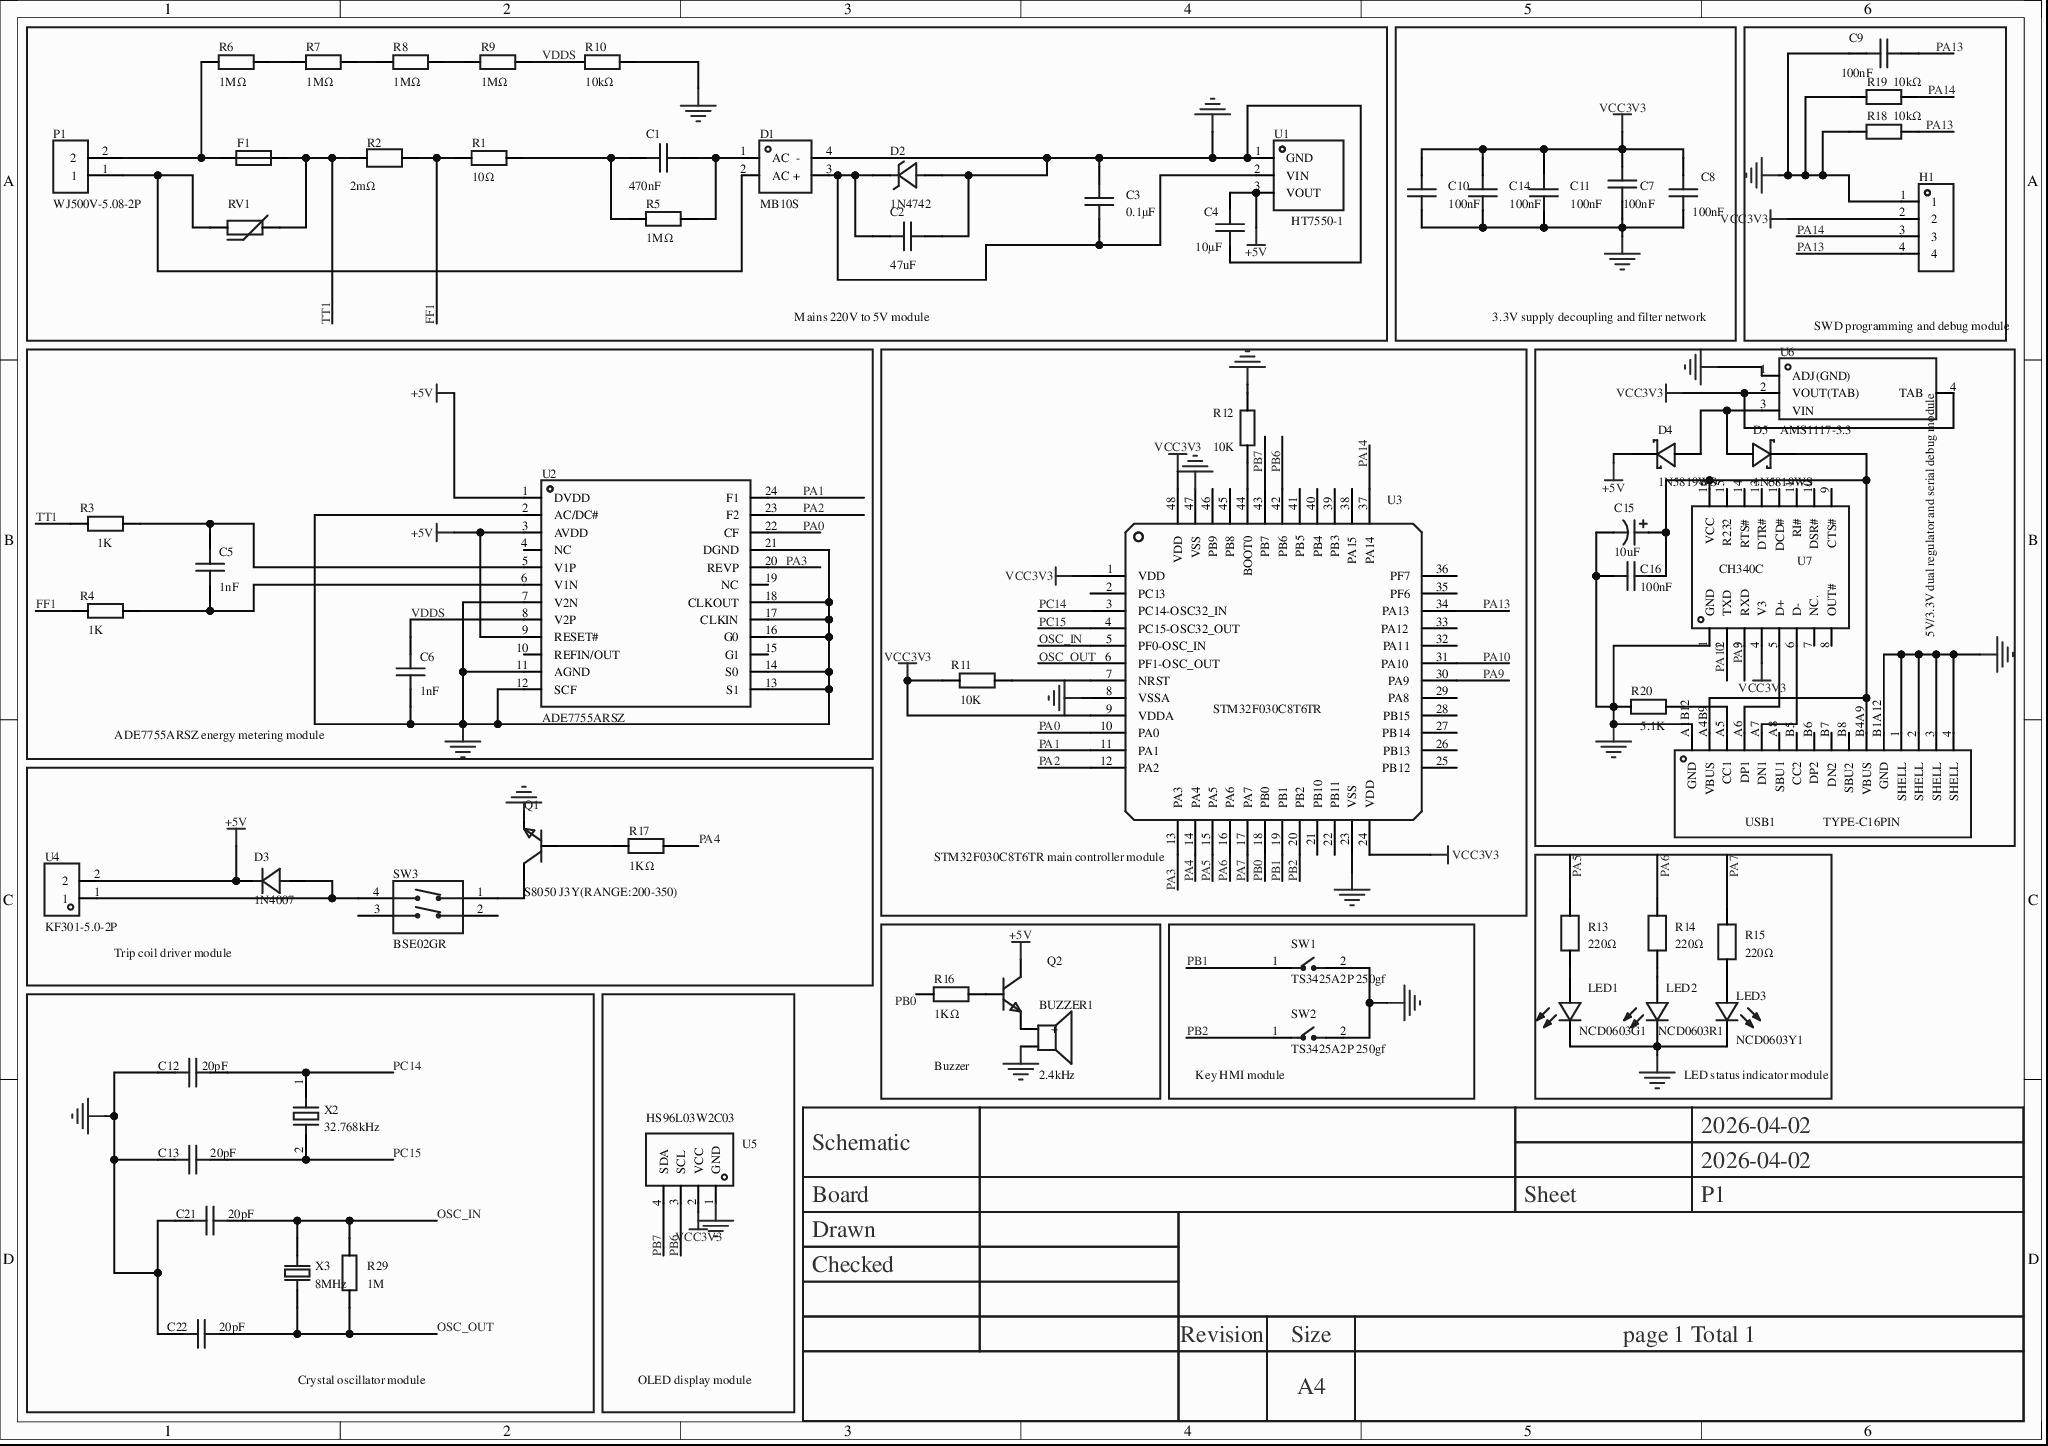
[diagram p0: MISC61242-3.schdoc]
# Altium project MISC61242-2.PrjPcb
1 sheet, 67 parts. Net scope: global (net labels, ports and power ports of the same name join across sheets).
Board file: MISC61242.pcbdoc

## Sheet MISC61242-3.schdoc
size 297 x 209 mm; Version: V1.0; @Project Name: MISC61242; @Update Date: 2026-04-13; @Create Date: 2026-04-13; @Board Name: MISC61242; @Create Time: 14:55:17; @Page Count: 1; @Page No: 1; @Schematic Name: MISC61242; @Update Time: 14:55:17; Size: A4

### Parts
BUZZER1  2.4kHz  [BUZ-TH_BD12.0-P7.60-D0.6-FD]
C1  470nF  [CAP-TH_L17.0-W5.5-P15.00-D1.2]
C2  47uF  [C0603]
C3  0.1μF  [C0603]
C4  10μF  [C0603]
C5  1nF  [C0603]
C6  1nF  [C0603]
C7  100nF  [C0805]
C8  100nF  [C0805]
C9  100nF  [C0603]
C10  100nF  [C0805]
C11  100nF  [C0603]
C12  20pF  [C0805]
C13  20pF  [C0805]
C14  100nF  [C0805]
C15  10uF  [CAP-SMD_BD5.0-L5.3-W5.3-FD]
C16  100nF  [C0603]
C21  20pF  [C0805]
C22  20pF  [C0805]
D1  MB10S  [MBS_L4.7-W4.0-P2.50-LS7.0-TL]
D2  1N4742  [DO-41_BD2.4-L4.7-P8.70-D0.8-FD]
D3  1N4007  [SMA_L4.3-W2.5-LS5.0-RD]
D4  1N5819WS  [SOD-323_L1.8-W1.3-LS2.5-RD]
D5  1N5819WS  [SOD-323_L1.8-W1.3-LS2.5-RD]
F1  2F.0500212000S1B02  [FUSE-TH_BD3.0-L7.2-P11.20-D0.6]  (value not drawn)
H1  (no value)  [HDR-TH_4P-P2.54-V-F]
LED1  NCD0603G1  [LED0603-RD_1]
LED2  NCD0603R1  [LED0603-RD_RED]
LED3  NCD0603Y1  [LED0603-RD]
P1  WJ500V-5.08-2P  [CONN-TH_2P-P5.00_WJ500V-5.08-2P]
Q1  S8050 J3Y(RANGE:200-350)  [SOT-23-3_L3.0-W1.7-P0.95-LS2.9-BR]
Q2  (no value)  [S8050_SOT-23]
R1  10Ω  [R0603]
R2  2mΩ  [RES-SMD_L6.4-W3.2-1]
R3  1K  [R0603]
R4  1K  [R0603]
R5  1MΩ  [R0603]
R6  1MΩ  [R1206]
R7  1MΩ  [R1206]
R8  1MΩ  [R1206]
R9  1MΩ  [R1206]
R10  10kΩ  [R0805]
R11  10K  [R0603]
R12  10K  [R0603]
R13  220Ω  [R0402]
R14  220Ω  [R0402]
R15  220Ω  [R0402]
R16  1KΩ  [R0603]
R17  1KΩ  [R0603]
R18  10kΩ  [R0805]
R19  10kΩ  [R0805]
R20  5.1K  [R0603]
R29  1M  [R0805]
RV1  190pF@1kHz  [RES-TH_L12.5-W6.7-P7.50-D1.2]  (value not drawn)
SW1  TS3425A2P 250gf  [SW-SMD_L3.9-W2.9-LS5.0]
SW2  TS3425A2P 250gf  [SW-SMD_L3.9-W2.9-LS5.0]
SW3  BSE02GR  [SW-TH_4P-L9.9-W6.8-P7.62-BL]
U1  HT7550-1  [SOT-89_L4.5-W2.5-P1.50-LS4.2-BR]
U2  ADE7755ARSZ  [SSOP-24_L8.1-W5.3-P0.65-LS7.8-BL]
U3  STM32F030C8T6TR  [LQFP-48_L7.0-W7.0-P0.50-LS9.0-BL]
U4  KF301-5.0-2P  [HDR-M-2.54_1X2]
U5  HS96L03W2C03  [OLED-TH_L27.8-W27.2-P2.54_C9900033791]
U6  AMS1117-3.3  [SOT-223-4_L6.5-W3.5-P2.30-LS7.0-BR]
U7  CH340C  [SOP-16_L10.0-W3.9-P1.27-LS6.0-BL]
USB1  TYPE-C16PIN  [USB-C-SMD_TYPE-C16PIN]
X2  32.768kHz  [CRYSTAL-SMD_L3.2-W1.5-FC-135R32.7680KF-A3]
X3  8MHz  [CRYSTAL-SMD_L3.2-W2.5_3225-8MHZ]

### Blocks framed on the sheet
Mains 220V to 5V module: C1-C4 D1 D2 F1 P1 R1 R2 R5-R10 RV1 U1
3.3V supply decoupling and filter network: C7 C8 C10 C11 C14
SWD programming and debug module: C9 H1 R18 R19
ADE7755ARSZ energy metering module: C5 C6 R3 R4 U2
STM32F030C8T6TR main controller module: R11 R12 U3
5V/3.3V dual regulator and serial debug module: C15 C16 D4 D5 R20 U6 U7 USB1
Trip coil driver module: D3 Q1 R17 SW3 U4
LED status indicator module: LED1-LED3 R13-R15
Buzzer: BUZZER1 Q2 R16
Key HMI module: SW1 SW2
Crystal oscillator module: C12 C13 C21 C22 R29 X2 X3
OLED display module: U5

### Nets
+5V: C4.2 D3.1(K) D4.1(K) Q2.3 U1.3(VOUT) U2.1(DVDD) U2.3(AVDD) U2.9(RESET#) U4.2
GND: BUZZER1.2 C2.2 C3.2 C4.1 C6.1 C7.2 C8.1 C9.1 C10.2 C11.1 C12.2 C13.1 C14.1 C15.2 C16.1 C21.1 C22.1 D1.4(-) D2.1(A) H1.1 LED1.1(K) LED2.1(K) LED3.1(K) Q1.2(E) R10.2 R12.2 R18.2 R19.2 R20.2 SW1.2 SW2.2 U1.1(GND) U2.2(AC/DC#) U2.7(V2N) U2.11(AGND) U2.12(SCF) U2.13(S1) U2.14(S0) U2.16(G0) U2.17(CLKIN) U2.18(CLKOUT) U2.21(DGND) U3.8(VSSA) U3.23(VSS) U3.47(VSS) U5.1(GND) U6.1(ADJ(GND)) U7.1(GND) USB1.1(SHELL) USB1.2(SHELL) USB1.3(SHELL) USB1.4(SHELL) USB1.A1B12(GND) USB1.B1A12(GND)
VCC3V3: C7.1 C8.2 C10.1 C11.2 C14.2 H1.2 R11.1 U3.1(VDD) U3.9(VDDA) U3.24(VDD) U3.48(VDD) U5.2(VCC) U6.2(VOUT(TAB)) U6.4(TAB) U7.4(V3)
FF1: R1.1 R2.2 R4.1
OSC_IN: C21.2 R29.2 U3.5(PF0-OSC_IN) X3.2
OSC_OUT: C22.2 R29.1 U3.6(PF1-OSC_OUT) X3.1
PA0: U2.22(CF) U3.10(PA0)
PA1: U2.24(F1) U3.11(PA1)
PA2: U2.23(F2) U3.12(PA2)
PA3: U2.20(REVP) U3.13(PA3)
PA4: R17.1 U3.14(PA4)
PA5: R13.2 U3.15(PA5)
PA6: R14.2 U3.16(PA6)
PA7: R15.2 U3.17(PA7)
PA9: U3.30(PA9) U7.3(RXD)
PA10: U3.31(PA10) U7.2(TXD)
PA13: C9.2 H1.4 R18.1 U3.34(PA13)
PA14: H1.3 R19.1 U3.37(PA14)
PB0: R16.2 U3.18(PB0)
PB1: SW1.1 U3.19(PB1)
PB2: SW2.1 U3.20(PB2)
PB6: U3.42(PB6) U5.3(SCL)
PB7: U3.43(PB7) U5.4(SDA)
PC14: C12.1 U3.3(PC14-OSC32_IN) X2.1
PC15: C13.2 U3.4(PC15-OSC32_OUT) X2.2(GND)
TT1: F1.2 R2.1 R3.1 RV1.2
VDDS: C6.2 R9.2 R10.1 U2.8(V2P)
NetBUZZER1_1: BUZZER1.1(+) Q2.2
NetC1_1: C1.1 D1.1(AC) R5.2
NetC1_2: C1.2 R1.2 R5.1
NetC2_1: C2.1 C3.1 D1.3(+) D2.2(K) U1.2(VIN)
NetC5_1: C5.1 R4.2 U2.6(V1N)
NetC5_2: C5.2 R3.2 U2.5(V1P)
NetC15_1: C15.1 C16.2 D5.1(K) U7.16(VCC) USB1.A4B9(VBUS) USB1.B4A9(VBUS)
NetD1_2: D1.2(AC) P1.1 RV1.1
NetD3_2: D3.2(A) SW3.4 U4.1
NetD4_2: D4.2(A) D5.2(A) U6.3(VIN)
NetF1_1: F1.1 P1.2 R6.1
NetLED1_2: LED1.2(A) R13.1
NetLED2_2: LED2.2(A) R14.1
NetLED3_2: LED3.2(A) R15.1
NetQ1_1: Q1.1(B) R17.2
NetQ1_3: Q1.3(C) SW3.1
NetQ2_1: Q2.1 R16.1
NetR6_2: R6.2 R7.1
NetR7_2: R7.2 R8.1
NetR8_2: R8.2 R9.1
NetR11_2: R11.2 U3.7(NRST)
NetR12_1: R12.1 U3.44(BOOT0)
NetR20_1: R20.1 USB1.A5(CC1)
NetU7_5: U7.5(D+) USB1.A6(DP1)
NetU7_6: U7.6(D-) USB1.A7(DN1)

Not connected (* = marked no-connect by the designer): SW3 2* 3*; U2 4(NC)* 10(REFIN/OUT)* 15(G1)* 19(NC)*; U3 2(PC13)* 21(PB10)* 22(PB11)* 25(PB12)* 26(PB13)* 27(PB14)* 28(PB15)* 29(PA8)* 32(PA11)* 33(PA12)* 35(PF6)* 36(PF7)* 38(PA15)* 39(PB3)* 40(PB4)* 41(PB5)* 45(PB8)* 46(PB9)*; U7 7(NC.)* 8(OUT#)* 9(CTS#)* 10(DSR#)* 11(RI#)* 12(DCD#)* 13(DTR#)* 14(RTS#)* 15(R232)*; USB1 A8(SBU1)* B5(CC2)* B6(DP2)* B7(DN2)* B8(SBU2)*

### Notes on the sheet
- 2026-04-02
- Schematic
- Board
- Sheet
- P1
- Drawn
- Checked
- Revision
- Size
- A4
- page 1 Total 1

### Library data of the parts
BUZZER1 = TMB12A05_C96093: Drive method: Active (with built-in driver circuit); Construction type: Electromagnetic; Rated voltage: 5V; Frequency: 2.4kHz; Sound pressure (SPL): 85dB;; Manufacturer: 华能; Voltage - Supply: 4V~8V; Current Consumption: 30mA; 3D Model: 16ab50e14c5b4f2c986c135bdba60e370819f05c4eef4c71ace90d822a990e87; 3D Model Transform: 472.44,472.176,0,90,0,0,-0.787,0,-177.165; AddInBom: yes; ModelName: BUZ-TH_D12.0-H9.5-P7.60; Device: TMB12A05_C96093; Symbol: TMB12A05; LCSC Part Name: 有源(内含驱动线路) 电磁式 2.4kHz; Supplier Part: C96093; Manufacturer Part: TMB12A05; Supplier Footprint: 插件,D=12mm; JLCPCB Part Class: Extended Part; Datasheet: https://item.szlcsc.com/datasheet/TMB12A05/97297.html; Supplier: LCSC; Driver Circuitry: Active (with built-in driver circuit); Technology: Electromagnetic; Voltage Rating: 5V; Value: 2.4kHz; Sound Pressure Level(SPL): 85dB; Diameter(φD): 12mm; Length: -; Width: -; Height: 9.8mm; Operating Temperature: -40℃~+85℃; FootprintName: BUZ-TH_BD12.0-P7.60-D0.6-FD; ConvertToPcb: yes
C1 = CBB21-400V474JP15: Capacitance: 470nF; Tolerance: ±5%; Rated voltage: 400V; Operating temperature: -40℃~+105℃;; Manufacturer: 东通电子; AddInBom: yes; ModelId: f8cf251704e9467493657d330e769cf70819f05c4eef4c71ace90d822a990e87; ModelName: CAP-TH_L17.0-W5.5-H10.0-P15.0; ModelTransform: 669.29,216.535,0,0,0,0,0,0,-137.795; Device: CBB21-400V474JP15; Symbol: CBB21-400V474JP15; FootprintName: CAP-TH_L17.0-W5.5-P15.00-D1.2; LCSC Part Name: 470nF ±5% 400V; SupplierPart: C2888194; ManufacturerPart: CBB21-400V474JP15; Supplier Footprint: 插件,P=15mm; JLCPCB Part Class: Extended Part; Datasheet: https://item.szlcsc.com/datasheet/CBB21-400V474JP15/3107607.html; Supplier: LCSC; ConvertToPcb: yes; Value: 470nF; Voltage Rating: 400V; Operating Temperature: -40℃~+105℃
C2 = CL10A476MQ8QRNC: Capacitance: 47uF; Tolerance: ±20%; Rated voltage: 6.3V; Temperature coefficient: X5R;; Manufacturer: SAMSUNG(三星); AddInBom: yes; ModelId: ac125912035d415993ca9572d50418b10819f05c4eef4c71ace90d822a990e87; ModelName: C0603_L1.6-W0.8-H0.8; ModelTransform: 62.992,31.496,0,0,0,0,0,0,0; Device: CL10A476MQ8QRNC; Symbol: CL10A476MQ8QRNC; FootprintName: C0603; LCSC Part Name: 47uF ±20% 6.3V; SupplierPart: C730416; ManufacturerPart: CL10A476MQ8QRNC; Supplier Footprint: 0603; JLCPCB Part Class: Extended Part; Datasheet: https://item.szlcsc.com/datasheet/CL10A476MQ8QRNC/778815.html; Supplier: LCSC; ConvertToPcb: yes; Value: 47uF; Voltage Rating: 6.3V; Temperature Coefficient: X5R
C3-C6 C11 = CAP_0603: Symbol: Capacitance; 3D Model: ac125912035d415993ca9572d50418b10819f05c4eef4c71ace90d822a990e87; 3D Model Transform: 62.992,31.496,0,0,0,0,0,0,0; ConvertToPcb: yes; ModelName: C0603_L1.6-W0.8-H0.8; Device: CAP_0603; Supplier Footprint: 0603; FootprintName: C0603; AddInBom: yes
  C3: Value: 0.1μF
  C4: Value: 10μF
  C5 C6: Value: 1nF
  C11: Value: 100nF
C7 C10 = GRM21BR71H104KA01L: Capacitance: 100nF; Tolerance: ±10%; Rated voltage: 50V; Temperature coefficient: X7R;; Manufacturer: muRata(村田); AddInBom: yes; ModelId: 1ba041120af144c991958decab20d2410819f05c4eef4c71ace90d822a990e87; ModelName: C0805_L2.0-W1.3-H1.3; ModelTransform: 78.74,51.181,0,0,0,0,0,0.0005,0; Device: GRM21BR71H104KA01L; Symbol: GRM21BR71H104KA01L; FootprintName: C0805; LCSC Part Name: 100nF ±10% 50V; SupplierPart: C77082; ManufacturerPart: GRM21BR71H104KA01L; Supplier Footprint: 0805; JLCPCB Part Class: Extended Part; Datasheet: https://item.szlcsc.com/datasheet/GRM21BR71H104KA01L/78209.html; Supplier: LCSC; ConvertToPcb: yes; Value: 100nF; Voltage Rating: 50V; Temperature Coefficient: X7R
C8 C14 = GRM21BR71H104KA01L: Capacitance: 100nF; Tolerance: ±10%; Rated voltage: 50V; Temperature coefficient: X7R;; Manufacturer: muRata(村田); 3D Model: 1ba041120af144c991958decab20d2410819f05c4eef4c71ace90d822a990e87; 3D Model Transform: 78.74,51.181,0,0,0,0,0,0.0005,0; AddInBom: yes; ModelName: C0805_L2.0-W1.3-H1.3; Device: GRM21BR71H104KA01L; Symbol: GRM21BR71H104KA01L; LCSC Part Name: 100nF ±10% 50V; Supplier Part: C77082; Manufacturer Part: GRM21BR71H104KA01L; Supplier Footprint: 0805; JLCPCB Part Class: Extended Part; Datasheet: https://item.szlcsc.com/datasheet/GRM21BR71H104KA01L/78209.html; Supplier: LCSC; Value: 100nF; Voltage Rating: 50V; Temperature Coefficient: X7R; FootprintName: C0805; ConvertToPcb: yes
C9 = FCC0603B104K500CT: Capacitance: 100nF; Tolerance: ±10%; Rated voltage: 50V; Temperature coefficient: X7R;; Manufacturer: FOJAN(富捷); AddInBom: yes; ModelId: ac125912035d415993ca9572d50418b10819f05c4eef4c71ace90d822a990e87; ModelName: C0603_L1.6-W0.8-H0.8; ModelTransform: 62.992,31.496,0,0,0,0,0,0,0; Device: FCC0603B104K500CT; Symbol: FCC0603B104K500CT; FootprintName: C0603; LCSC Part Name: 100nF ±10% 50V; SupplierPart: C5137636; ManufacturerPart: FCC0603B104K500CT; Supplier Footprint: 0603; JLCPCB Part Class: Extended Part; Datasheet: https://item.szlcsc.com/datasheet/FCC0603B104K500CT/5747088.html; Supplier: LCSC; ConvertToPcb: yes; Value: 100nF; Voltage Rating: 50V; Temperature Coefficient: X7R
C12 C13 C21 C22 = CAP_0805: Symbol: CapAcitance; 3D Model: 1ba041120af144c991958decab20d241; 3D Model Transform: 78.74,51.181,0,0,0,0,0,0.0005,0; ConvertToPcb: yes; ModelName: C0805_L2.0-W1.3-H1.3; Device: CAP_0805; Value: 20pF; Supplier Footprint: 0805; FootprintName: C0805; AddInBom: yes
C15 = RST10UF50V016: Capacitance: 10uF; Tolerance: ±20%; Rated voltage: 50V; Ripple current: 24mA@120Hz; Equivalent series resistance (ESR): -;; Manufacturer: KNSCHA(科尼盛); AddInBom: yes; Lifetime: 2000hrs@105℃; ModelId: 16f5696d655347d6a4362817d02ce59a0819f05c4eef4c71ace90d822a990e87; ModelName: CAP-SMD_BD5.0-L5.3-W5.3-LS5.5-FD; ModelTransform: 216.535,208.661,0,0,0,0,0,0,0; Device: RST10UF50V016; Symbol: RST10UF50V016; FootprintName: CAP-SMD_BD5.0-L5.3-W5.3-FD; LCSC Part Name: 10uF ±20% 50V; SupplierPart: C4747971; ManufacturerPart: RST10UF50V016; Supplier Footprint: SMD,D5xL5.4mm; JLCPCB Part Class: Extended Part; Datasheet: https://atta.szlcsc.com/upload/public/pdf/source/20220722/47144637C831FC4476CE4962252D8002.pdf; Supplier: LCSC; ConvertToPcb: yes; Value: 10uF; Voltage Rating: 50V; Ripple Current: 24mA@120Hz; Equivalent Series Resistance(ESR): -; Diameter: 5mm; Height - Seated (Max): 5.4mm; Operating Temperature: -40℃~+105℃
C16 = CGA0603X7R104K500JT: Capacitance: 100nF; Tolerance: ±10%; Rated voltage: 50V; Temperature coefficient: X7R;; Manufacturer: HRE(芯声); AddInBom: yes; ModelId: ac125912035d415993ca9572d50418b10819f05c4eef4c71ace90d822a990e87; ModelName: C0603_L1.6-W0.8-H0.8; ModelTransform: 62.992,31.496,0,0,0,0,0,0,0; Device: CGA0603X7R104K500JT; Symbol: CGA0603X7R104K500JT; FootprintName: C0603; LCSC Part Name: 100nF ±10% 50V; SupplierPart: C6119867; ManufacturerPart: CGA0603X7R104K500JT; Supplier Footprint: 0603; JLCPCB Part Class: Extended Part; Datasheet: https://item.szlcsc.com/datasheet/CGA0603X7R104K500JT/7062573.html; Supplier: LCSC; ConvertToPcb: yes; Value: 100nF; Voltage Rating: 50V; Temperature Coefficient: X7R
D1 = MB10S_C42463381: Forward voltage (Vf): 1.1V@1A; DC reverse voltage (Vr): 1kV; Rectified current: 1A; Non-repetitive peak surge current (Ifsm): 35A;; Manufacturer: R+O(宏嘉诚); AddInBom: yes; Reverse Leakage Current (Ir): 5uA; Operating Junction Temperature Range: -55℃~+150℃; ModelId: 7dad5ddbf7424b73bca0092e0c7e32040819f05c4eef4c71ace90d822a990e87; ModelName: MBS_L4.7-W4.0-H2.5-LS7.0; ModelTransform: 185.039,275.591,0,270,0,0,0,0,0; Device: MB10S_C42463381; Symbol: MB10S_C42463381; FootprintName: MBS_L4.7-W4.0-P2.50-LS7.0-TL; LCSC Part Name: 耐压:1000V 电流:1A; SupplierPart: C42463381; ManufacturerPart: MB10S; Supplier Footprint: MBS; JLCPCB Part Class: Extended Part; Datasheet: https://item.szlcsc.com/datasheet/MB10S/44554700.html; Supplier: LCSC; ConvertToPcb: yes; Voltage - Forward(Vf@If): 1.1V@1A; Voltage - DC Reverse(Vr): 1kV; Current - Rectified: 1A; Non-Repetitive Peak Forward Surge Current: 35A
D2 = 1N4742: Diode configuration: Single; Zener voltage (nominal): 12V; Zener voltage (range): 11.45V~12.95V; Power dissipation (Pd): 1W;; Manufacturer: LGE(鲁光); AddInBom: yes; Reverse Leakage Current (Ir): 5uA; Impedance(Zzt): 9Ω; Impedance(Zzk): 700Ω; ModelId: 6de1e9b71a0d4751b4e9df530304c1a30819f05c4eef4c71ace90d822a990e87; ModelName: DO-41_D2.4-L4.7-P8.70; ModelTransform: 374.015,94.428,0,180,0,0,0,0,-137.795; Device: 1N4742; Symbol: 1N4742; FootprintName: DO-41_BD2.4-L4.7-P8.70-D0.8-FD; LCSC Part Name: 独立式 耐压:12V 电流:5uA; SupplierPart: C5174492; ManufacturerPart: 1N4742; Supplier Footprint: DO-41; JLCPCB Part Class: Extended Part; Datasheet: https://item.szlcsc.com/datasheet/1N4742/5826851.html; Supplier: LCSC; ConvertToPcb: yes; Diode Configuration: Single; Zener Voltage(Nom): 12V; Zener Voltage(Range): 11.45V~12.95V; Pd - Power Dissipation: 1W
D3 = 1N4007_C727081: Diode configuration: Single; Forward voltage (Vf): 1.1V@1A; DC reverse voltage (Vr): 1kV; Rectified current: 1A;; Manufacturer: TWGMC(迪嘉); AddInBom: yes; Reverse Leakage Current (Ir): 5uA; ModelId: 5b53cc1b87a148cc9fa13125be89f9480819f05c4eef4c71ace90d822a990e87; ModelTransform: 194.8815,98.425,0,0,0,0,0,0,0; Device: 1N4007_C727081; Symbol: 1N4007_C727081; FootprintName: SMA_L4.3-W2.5-LS5.0-RD; LCSC Part Name: 1N4007; SupplierPart: C727081; ManufacturerPart: 1N4007; Supplier Footprint: SMA(DO-214AC); JLCPCB Part Class: Extended Part; Datasheet: https://item.szlcsc.com/datasheet/1N4007/774186.html; Supplier: LCSC; ConvertToPcb: yes; Diode Configuration: Single; Voltage - Forward(Vf@If): 1.1V@1A; Voltage - DC Reverse(Vr): 1kV; Current - Rectified: 1A; ModelName: SMA_L4.3-W2.5-LS5.0-RD
D4 D5 = 1N5819WS_C191023: Forward voltage (Vf): 600mV@1A; DC reverse voltage (Vr): 40V; Rectified current: 1A;; Manufacturer: Hottech(合科泰); AddInBom: yes; Non-Repetitive Peak Forward Surge Current: 25A; ModelId: db63db13d9e342eb939127d413d6200b0819f05c4eef4c71ace90d822a990e87; ModelTransform: 104.3305,51.181,0,0,0,0,0,0,0; Device: 1N5819WS_C191023; Symbol: 1N5819WS; FootprintName: SOD-323_L1.8-W1.3-LS2.5-RD; LCSC Part Name: 电压:40V 电流:1A; SupplierPart: C191023; ManufacturerPart: 1N5819WS; Supplier Footprint: SOD-323; JLCPCB Part Class: Basic Part; Datasheet: https://item.szlcsc.com/datasheet/1N5819WS/213850.html; Supplier: LCSC; ConvertToPcb: yes; Voltage - Forward(Vf@If): 600mV@1A; Voltage - DC Reverse(Vr): 40V; Current - Rectified: 1A; ModelName: SOD-323_L1.8-W1.3-LS2.5-RD
F1 = 2F.0500212000S1B02: Type: glass tube fuse; Rated current: 500mA; Rated voltage (AC): 250V; 125V; Breaking capacity: 50A;; Manufacturer: xcfuse(旭程); Symbol: 2F500MA 250V; AddInBom: yes; Voltage Rating (AC): 250V；125V; Melting I2t: 0.1; ModelId: 8493180d87ef424b8637a2753ca991c60819f05c4eef4c71ace90d822a990e87; ModelName: FUSE-TH_BD3.4-L7.1-P11.20-D0.6; ModelTransform: 497.6368,134.6891,0,0,0,0,0,0,-196.85; Device: 2F.0500212000S1B02; FootprintName: FUSE-TH_BD3.0-L7.2-P11.20-D0.6; LCSC Part Name: 插件式保险丝; SupplierPart: C140536; ManufacturerPart: 2F.0500212000S1B02; Supplier Footprint: 插件,D2.7xL7.3mm; JLCPCB Part Class: Extended Part; Datasheet: https://item.szlcsc.com/datasheet/2F.0500212000S1B02/151862.html; Supplier: LCSC; ConvertToPcb: yes; Type: Glass tube fuse; Current Rating: 500mA; Operating Temperature: -40℃~+125℃; Interrupt Rating: 50A; Diameter (φD): 2.7mm; Length: 7.3mm
H1 = HDR-F_2.54_1x4P: Symbol: 2.54-1*4P female; ConvertToPcb: yes; ModelId: d187812051054f85879fcaa51a310d8e0819f05c4eef4c71ace90d822a990e87; ModelTransform: 419.6842,98.464,0,0,0,0,0,0,-118.11; Device: HDR-F_2.54_1x4P; FootprintName: HDR-TH_4P-P2.54-V-F; AddInBom: yes; SupplierPart: C2718488; Supplier Footprint: 插件; ModelName: HDR-TH_4P-P2.54-V-F
LED1 = NCD0603G1: Lamp head type: -; Emitting color: Emerald green; Forward voltage (Vf): 2.6V~3.6V; Power: 72mW; Forward current: 20mA; Wavelength: 515nm~530nm; Diode configuration: Single diode; Lens color: -; Color temperature: -; Luminous intensity: 900mcd; Viewing angle: 130°; Tape packing: -; Operating temperature: -30℃~+85℃;; Manufacturer: 国星光电; Symbol: FC-D1608UGK-520D10; Add into BOM: yes; 3D Model: 3beb0148d24d477aac1d9f7d4b6d534c; 3D Model Transform: 62.2046,31.496,0,0,0,0,-1.948,0.215,0; Peak Wavelength: 520nm; Device: NCD0603G1; Convert to PCB: yes; LCSC Part Name: 片式发光二极管; Supplier Part: C84267; Manufacturer Part: NCD0603G1; Supplier Footprint: 0603; JLCPCB Part Class: Extended Part; Datasheet: https://item.szlcsc.com/datasheet/NCD0603G1/85436.html; Supplier: LCSC; Lamp Holder Type: -; Illumination Color: Emerald green; Voltage - Forward(Vf): 2.6V~3.6V; Power(Watts): 72mW; Forward Current: 20mA; Wavelength - Dominant: 515nm~530nm; Diode Configuration: Single diode; Lens Color: -; Color Temperature: -; Luminous Intensity: 900mcd; Viewing Angle: 130°; Mounting Style: -; Operating Temperature: -30℃~+85℃; FootprintName: LED0603-RD_1; ModelName: LED0603-RD_1
LED2 = NCD0603R1_C84263: Lamp head type: -; Emitting color: Red; Forward voltage (Vf): 1.6V~2.6V; Power: 65mW; Forward current: 25mA; Wavelength: 615nm~630nm; Diode configuration: Single diode; Lens color: -; Color temperature: -; Luminous intensity: 220mcd; Viewing angle: 130°; Tape packing: -; Operating temperature: -30℃~+85℃;; Manufacturer: 国星光电; Symbol: FC-DA1608HRK-620D; AddInBom: yes; Peak Wavelength: 630nm; ModelId: 74041d3a270d435c8600a9ab9b7641c00819f05c4eef4c71ace90d822a990e87; ModelTransform: 63.7794,31.496,0,0,0,0,0,-0.002,0; Device: NCD0603R1_C84263; FootprintName: LED0603-RD_RED; LCSC Part Name: 片式发光二极管; SupplierPart: C84263; ManufacturerPart: NCD0603R1; Supplier Footprint: 0603; JLCPCB Part Class: Extended Part; Datasheet: https://item.szlcsc.com/datasheet/NCD0603R1/85432.html; Supplier: LCSC; ConvertToPcb: yes; Lamp Holder Type: -; Illumination Color: Red; Voltage - Forward(Vf): 1.6V~2.6V; Power(Watts): 65mW; Forward Current: 25mA; Wavelength - Dominant: 615nm~630nm; Diode Configuration: Single diode; Lens Color: -; Color Temperature: -; Luminous Intensity: 220mcd; Viewing Angle: 130°; Mounting Style: -; Operating Temperature: -30℃~+85℃; ModelName: LED0603-RD_RED
LED3 = NCD0603Y1: Lamp head type: -; Emitting color: Yellow; Forward voltage (Vf): 1.6V~2.6V; Power: 65mW; Forward current: 25mA; Wavelength: 586nm~595nm; Diode configuration: Single diode; Lens color: -; Color temperature: -; Luminous intensity: 220mcd; Viewing angle: 130°; Tape packing: -; Operating temperature: -30℃~+85℃;; Manufacturer: 国星光电; Symbol: FC-D1608HYK-588J; AddInBom: yes; Peak Wavelength: 595nm; ModelId: 1f0d29a91be547639d425604e9b96ebb0819f05c4eef4c71ace90d822a990e87; ModelTransform: 63.7794,32.283,0,0,0,0,0,0,0; Device: NCD0603Y1; FootprintName: LED0603-RD; LCSC Part Name: 片式发光二极管; SupplierPart: C84268; ManufacturerPart: NCD0603Y1; Supplier Footprint: 0603; JLCPCB Part Class: Extended Part; Datasheet: https://item.szlcsc.com/datasheet/NCD0603Y1/85437.html; Supplier: LCSC; ConvertToPcb: yes; Lamp Holder Type: -; Illumination Color: Yellow; Voltage - Forward(Vf): 1.6V~2.6V; Power(Watts): 65mW; Forward Current: 25mA; Wavelength - Dominant: 586nm~595nm; Diode Configuration: Single diode; Lens Color: -; Color Temperature: -; Luminous Intensity: 220mcd; Viewing Angle: 130°; Mounting Style: -; Operating Temperature: -30℃~+85℃; ModelName: LED0603-RD
P1 = WJ500V-5.08-2P: Structure: 1x2P; Pitch: 5.08mm; Color: Green; Mounting: Through-hole; Rated current: 18A; Rated voltage: 250V; Rows: 1; Wire gauge - AWG: 14~30; Wire gauge - mm²: 2.5; Pins per row: 2; Contact material: -; Contact plating: -; Operating temperature range: -40℃~+105℃; Soldering temperature (max.): -;; Manufacturer: KANGNEX(康奈克斯电气); Symbol: WJ500V-5.08-2P-14-00A; AddInBom: yes; Wire Gauge - mm2: 2.5; Number of PINs Per Row: 2; Screw Specification: M2.5; ModelId: 0f4a503c8d3b4ae19ed61267f5e9a1d70819f05c4eef4c71ace90d822a990e87; ModelTransform: 423.621,393.7,0,0,0,0,-11.811,19.685,-137.795; Device: WJ500V-5.08-2P; FootprintName: CONN-TH_2P-P5.00_WJ500V-5.08-2P; LCSC Part Name: 1x2P 5.08mm 直插 排数:1 每排P数:2; SupplierPart: C8465; ManufacturerPart: WJ500V-5.08-2P; Supplier Footprint: 插件,P=5.08mm; JLCPCB Part Class: Extended Part; Datasheet: https://atta.szlcsc.com/upload/public/pdf/source/20191225/C8465_02D34CE5B5B4A53DF5891601D97FA9F4.pdf; Supplier: LCSC; ConvertToPcb: yes; Mounting Style: Through-hole; Current Rating (Max): 18A; Voltage Rating (Max): 250V; Number of Pins: 2P; Number of Rows: 1; Wire Gauge - AWG: 14~30; Contact Material: -; Contact Plating: -; Operating Temperature Range: -40℃~+105℃; Soldering Temperature(Max): -; ModelName: CONN-TH_2P-P5.00_WJ500V-5.08-2P
Q1 = S8050 J3Y(RANGE:200-350): Transistor type: NPN; Collector current (Ic): 500mA; Collector-emitter breakdown voltage (Vceo): 25V; Power dissipation (Pd): 300mW; DC current gain (hFE): 200@500mA,1V;; Manufacturer: CJ(江苏长电/长晶); Symbol: S8050_C2146; AddInBom: yes; Transition frequency(fT): 150MHz; Current - Collector Cutoff: 100nA; Vce Saturation(VCE(sat)): 600mV@500mA,50mA; Emitter-Base Voltage(Vebo): 5V; Number: 1 NPN; ModelId: 89cb27a44ab2466697082bb9fd73a7d00819f05c4eef4c71ace90d822a990e87; ModelName: SOT-23-3L_L2.9-W1.6-H1.1-LS2.8-P0.95; ModelTransform: 114.173,110.236,0,90,0,0,0,0,0; Device: S8050 J3Y(RANGE:200-350); FootprintName: SOT-23-3_L3.0-W1.7-P0.95-LS2.9-BR; LCSC Part Name: H档(200-350) NPN 电流:0.5A 电压:25V; SupplierPart: C2146; ManufacturerPart: S8050 J3Y(RANGE:200-350); Supplier Footprint: SOT-23; JLCPCB Part Class: Basic Part; Datasheet: https://item.szlcsc.com/datasheet/S8050%2520J3Y(RANGE%253A200-350)/2503.html; Supplier: LCSC; ConvertToPcb: yes; type: NPN; Current - Collector(Ic): 500mA; Collector - Emitter Voltage VCEO: 25V; Pd - Power Dissipation: 300mW; DC Current Gain: 200@500mA,1V; Operating Temperature: -55℃~+150℃
Q2 = S8050_SOT_NPN: Symbol: NPN; ConvertToPcb: yes; ModelId: c62791f0466c4ae2a892c056b845b0ca0819f05c4eef4c71ace90d822a990e87; ModelName: SOT-23-3P_L2.9-W1.3-H1.0-LS2.4-P0.95; ModelTransform: 98.6,114.12,41.29,180,0,0,0,0,-3; Device: S8050_SOT_NPN; FootprintName: S8050_SOT-23; AddInBom: yes; Supplier Footprint: SOT-23
R1 R3-R5 R11 R12 R16 R17 = Res_0603: Symbol: Resistor; 3D Model: fc143cca1e79419f9cd78b61e9279f080819f05c4eef4c71ace90d822a990e87; 3D Model Transform: 31.8897,63.7794,0,90,0,0,0,0,0; ConvertToPcb: yes; Device: Res_0603; Supplier Footprint: 0603; FootprintName: R0603; AddInBom: yes; ModelName: R0603
  R1: Value: 10Ω
  R3 R4: Value: 1K
  R5: Value: 1MΩ
  R11 R12: Value: 10K
  R16 R17: Value: 1KΩ
R2 = HoLLR2512-3W-2mR-1%: Resistor type: Sense resistor; Resistance: 2mΩ; Tolerance: ±1%; Rated voltage drop: -; Power: 3W; Temperature coefficient: ±50ppm/℃; Mounting: SMD;; Manufacturer: Milliohm(毫欧); AddInBom: yes; Rated Current: 77.5A; ModelId: 2a92684014bd46c593e4aa7ce823c3500819f05c4eef4c71ace90d822a990e87; ModelTransform: 251.968,125.984,0,0,0,0,0,0,0; Device: HoLLR2512-3W-2mR-1%; Symbol: HOLLR2512-3W-2MR-1%; FootprintName: RES-SMD_L6.4-W3.2-1; LCSC Part Name: 2mΩ ±1% 3W; SupplierPart: C2994640; ManufacturerPart: HoLLR2512-3W-2mR-1%; Supplier Footprint: 2512; JLCPCB Part Class: Extended Part; Datasheet: https://atta.szlcsc.com/upload/public/pdf/source/20220330/9E8D3880B1628B3B70C68092C8A7E08B.pdf; Supplier: LCSC; ConvertToPcb: yes; Type: Sense resistor; Value: 2mΩ; Rated Output Voltage: -; Power(Watts): 3W; Temperature Coefficient: ±50ppm/℃; Mounting Sytle: SMD; ModelName: RES-SMD_L6.4-W3.2-1
R6-R9 = 1206W4F1004T5E: Resistor type: Thick-film resistor; Resistance: 1MΩ; Tolerance: ±1%; Power: 250mW; Operating voltage: 200V; Temperature coefficient: ±100ppm/℃;; Manufacturer: UNI-ROYAL(厚声); AddInBom: yes; ModelId: 89a1f13db2384da588040e0b3c55bf660819f05c4eef4c71ace90d822a990e87; ModelName: R1206_L3.2-W1.6-H0.6; ModelTransform: 125.984,62.992,0,0,0,0,0,0,0; Device: 1206W4F1004T5E; Symbol: 1206W4F1004T5E; FootprintName: R1206; LCSC Part Name: 1MΩ ±1% 250mW 厚膜电阻; SupplierPart: C17927; ManufacturerPart: 1206W4F1004T5E; Supplier Footprint: 1206; JLCPCB Part Class: Basic Part; Datasheet: https://item.szlcsc.com/datasheet/1206W4F1004T5E/18615.html; Supplier: LCSC; ConvertToPcb: yes; Type: Thick-film resistor; Value: 1MΩ; Power(Watts): 250mW; Voltage-Supply(Max): 200V; Temperature Coefficient: ±100ppm/℃; Operating Temperature: -55℃~+155℃
R10 R18 R19 = 0805W8F1002T5E_C17414: Resistor type: Thick-film resistor; Resistance: 10kΩ; Tolerance: ±1%; Power: 125mW; Operating voltage: 150V; Temperature coefficient: ±100ppm/℃;; Manufacturer: UNI-ROYAL(厚声); AddInBom: yes; ModelId: 37a81e68749a4138bd2dfa6897b24b850819f05c4eef4c71ace90d822a990e87; ModelName: R0805_L2.0-W1.3-H0.6; ModelTransform: 78.74,51.181,0,0,0,0,0,-0.0005,0; Device: 0805W8F1002T5E_C17414; Symbol: 0805W8F1002T5E; FootprintName: R0805; LCSC Part Name: 10kΩ ±1% 125mW 厚膜电阻; SupplierPart: C17414; ManufacturerPart: 0805W8F1002T5E; Supplier Footprint: 0805; JLCPCB Part Class: Basic Part; Datasheet: https://item.szlcsc.com/datasheet/0805W8F1002T5E/18102.html; Supplier: LCSC; ConvertToPcb: yes; Type: Thick-film resistor; Value: 10kΩ; Power(Watts): 125mW; Voltage-Supply(Max): 150V; Temperature Coefficient: ±100ppm/℃; Operating Temperature: -55℃~+155℃
R13-R15 = FRC0402F2200TS: Resistor type: Thick-film resistor; Resistance: 220Ω; Tolerance: ±1%; Power: 62.5mW; Operating voltage: 50V; Temperature coefficient: ±100ppm/℃;; Manufacturer: FOJAN(富捷); AddInBom: yes; ModelId: 98c88bc2b9094f218f3a3e30a70127380819f05c4eef4c71ace90d822a990e87; ModelName: R0402_L1.0-W0.5-H0.4; ModelTransform: 39.37,19.685,0,0,0,0,0,0,0; Device: FRC0402F2200TS; Symbol: FRC0402F2200TS; FootprintName: R0402; LCSC Part Name: 220Ω ±1% 62.5mW 厚膜电阻; SupplierPart: C2909336; ManufacturerPart: FRC0402F2200TS; Supplier Footprint: 0402; JLCPCB Part Class: Extended Part; Datasheet: https://item.szlcsc.com/datasheet/FRC0402F2200TS/3186271.html; Supplier: LCSC; ConvertToPcb: yes; Type: Thick-film resistor; Value: 220Ω; Power(Watts): 62.5mW; Voltage-Supply(Max): 50V; Temperature Coefficient: ±100ppm/℃; Operating Temperature: -55℃~+155℃
R20 = Res_0603: Symbol: Resistor; ConvertToPcb: yes; ModelId: fc143cca1e79419f9cd78b61e9279f080819f05c4eef4c71ace90d822a990e87; ModelTransform: 31.8897,63.7794,0,90,0,0,0,0,0; Device: Res_0603; Value: 5.1K; FootprintName: R0603; AddInBom: yes; Supplier Footprint: 0603; ModelName: R0603
R29 = Res_0805: Symbol: Resistor; 3D Model: 37a81e68749a4138bd2dfa6897b24b85; 3D Model Transform: 78.74,51.181,0,0,0,0,0,-0.0005,0; ConvertToPcb: yes; ModelName: R0805_L2.0-W1.3-H0.6; Device: Res_0805; Value: 1M; Supplier Footprint: 0805; FootprintName: R0805; AddInBom: yes
RV1 = 10D471K_C8760: Varistor voltage: 423V~517V; Clamping voltage: 775V; Operating voltage (DC): 385V; Operating voltage (AC): 300V;; Manufacturer: RUILON(瑞隆源); Symbol: 10D471K-C8760; AddInBom: yes; Peak Current: 2.5kA; Energy: 42.3J; Rated Wattage: 400mW; ModelId: fcca3f9494a74590ab8e2cf67301bbb60819f05c4eef4c71ace90d822a990e87; ModelName: RES-TH_L12.5-W6.7-P7.50-S6.3; ModelTransform: 492.075,271.653,0,0,0,0,0,0,-137.795; Device: 10D471K_C8760; FootprintName: RES-TH_L12.5-W6.7-P7.50-D1.2; LCSC Part Name: 钳位电压775V 42.3焦耳 插件压敏电阻; SupplierPart: C8760; ManufacturerPart: 10D471K; Supplier Footprint: 插件,P=7.5mm; JLCPCB Part Class: Extended Part; Datasheet: https://item.szlcsc.com/datasheet/10D471K/9271.html; Supplier: LCSC; ConvertToPcb: yes; Varistor Voltage: 423V~517V; Clamping Voltage: 775V; Maximum DC Volts: 385V; Maximum AC Volts: 300V; Value: 190pF@1kHz
SW1 SW2 = TS3425A2P 250gf: Circuit structure: SPST; Button shape: Round; Actuation force: 2.5N; Mounting: Upright SMD; Length: 3.9mm; Width: 2.9mm; Height: 2.5mm; Bracket: No bracket; Contact current: 50mA; Rated voltage: 12V; Lamp: None; Operating life: 5 ten-thousand cycles;; Manufacturer: SHOU HAN(首韩); AddInBom: yes; Actuator Style: Round button; Actuator/Cap Color: Black; ModelId: 284ae12b719245d9ac94bed245e30d2a0819f05c4eef4c71ace90d822a990e87; ModelTransform: 196.85,114.173,0,0,0,0,0,0,0; Device: TS3425A2P 250gf; Symbol: TS3425A2P 250GF; FootprintName: SW-SMD_L3.9-W2.9-LS5.0; LCSC Part Name: 正按小龟 3*4*2.5mm 两脚不带柱 250gf; SupplierPart: C7431069; ManufacturerPart: TS3425A2P 250gf; Supplier Footprint: SMD; JLCPCB Part Class: Extended Part; Datasheet: https://item.szlcsc.com/datasheet/TS3425A2P%2520250gf/8431421.html; Supplier: LCSC; ConvertToPcb: yes; Circuit: SPST; Operating Force: 2.5N; Mounting Type: Upright SMD; Switch Height: 2.5mm; with Bracket: No bracket; Contact Current: 50mA; Voltage Rating: 12V; With Lamp: None; Termination Style: SMD tab; Life: 5 ten-thousand cycles; Operating Temperature: -20℃~+70℃; ModelName: SW-SMD_L3.9-W2.9-LS5.0
SW3 = BSE02GR: Circuit structure: SPST; Number of positions: 2; Rated current: 25mA; Rated voltage: 24V; Operating life: 2 thousand cycles; Color: Red;; Manufacturer: BIWIN(百莹); AddInBom: yes; Number of Positions: 2 positions; ModelId: 63ebfb56372a4ceba18c0aed18e1c9250819f05c4eef4c71ace90d822a990e87; ModelTransform: 259.881,389.763,0,0,0,0,0,0,-153.543; Device: BSE02GR; Symbol: BSE02GR; FootprintName: SW-TH_4P-L9.9-W6.8-P7.62-BL; LCSC Part Name: 2.54mm间距2P 红色插件拨码开关; SupplierPart: C3294681; ManufacturerPart: BSE02GR; Supplier Footprint: 插件,P=2.54mm; JLCPCB Part Class: Extended Part; Datasheet: https://item.szlcsc.com/datasheet/BSE02GR/3859081.html; Supplier: LCSC; ConvertToPcb: yes; Circuit: SPST; Termination Style: -; Lead Pitch: 2.54mm; Current Rating: 25mA; Voltage Rating: 24V; Operating Temperature: -40℃~+80℃; Operating Life: 2 thousand cycles; Color: Red; ModelName: SW-TH_4P-L9.9-W6.8-P7.62-BL
U1 = HT7550-1_C347189: Output type: Fixed; Operating voltage: 30V; Output voltage: 5V; Output current: 100mA; Power supply rejection ratio (PSRR): -; Output polarity: Positive;; Manufacturer: UMW(友台半导体); 3D Model: 6db690b7897d4d18a30d90c1b89525ee0819f05c4eef4c71ace90d822a990e87; 3D Model Transform: 161.417,169.291,0,180,0,0,-12.745,0.006,0; Voltage Dropout: 100mV@(1mA); standby current: 3uA; Number of Outputs: 1; AddInBom: yes; ModelName: SOT-89-3_L4.3-W2.5-H1.6-LS4.1-P1.50; Device: HT7550-1_C347189; Symbol: HT7550-1_C347189; LCSC Part Name: 输入30V 输出5V 100mA; Supplier Part: C347189; Manufacturer Part: HT7550-1; Supplier Footprint: SOT-89; JLCPCB Part Class: Extended Part; Datasheet: https://item.szlcsc.com/datasheet/HT7550-1/323849.html; Supplier: LCSC; Output Type: Fixed; Voltage - Supply: 30V; Output Voltage: 5V; Output Current: 100mA; Power Supply Rejection Ratio (PSRR): -; Noise: -; Operating Temperature: -25℃~+70℃; Output Configuration: Positive; FootprintName: SOT-89_L4.5-W2.5-P1.50-LS4.2-BR; ConvertToPcb: yes
U2 = ADE7755ARSZ: Operating voltage: 4.75V~5.25V; Operating current: 3.5mA;; Manufacturer: ADI(亚德诺); 3D Model: f5b2473ce40e4151ba004f11ac5dda6c0819f05c4eef4c71ace90d822a990e87; 3D Model Transform: 322.834,307.086,0,0,0,0,0,0,0; Number of Channels: 2; Dynamic Range: 500:1; AddInBom: yes; ModelName: SSOP-24_L8.2-W5.3-H1.8-LS7.8-P0.65; Device: ADE7755ARSZ; Symbol: ADE7755ARSZ; LCSC Part Name: ADE7755 电能计量IC; Supplier Part: C1523825; Manufacturer Part: ADE7755ARSZ; Supplier Footprint: SSOP-24; JLCPCB Part Class: Extended Part; Datasheet: https://item.szlcsc.com/datasheet/ADE7755ARSZ/1614623.html; Supplier: LCSC; Voltage - Supply: 4.75V~5.25V; Current - Supply: 3.5mA; Operating Temperature: -40℃~+85℃; FootprintName: SSOP-24_L8.1-W5.3-P0.65-LS7.8-BL; ConvertToPcb: yes
U3 = STM32F030C8T6TR: CPU core: ARM-M0; CPU max. frequency: 48MHz; Application field: -;; Manufacturer: ST(意法半导体); AddInBom: yes; Program Storage Size: 64KB; Program Memory Type: FLASH; Number of I/O: 39; ADC (Bit): 12bit; Voltage - Supply: 2.4V~3.6V; ModelId: 093be70396ff421eb2cdb946d5311efc0819f05c4eef4c71ace90d822a990e87; ModelName: LQFP-48_L7.0-W7.0-H1.4-LS9.0-P0.50; ModelTransform: 354.331,354.331,0,0,0,0,0,0,0; Device: STM32F030C8T6TR; Symbol: STM32F030C8T6TR; FootprintName: LQFP-48_L7.0-W7.0-P0.50-LS9.0-BL; LCSC Part Name: 主流ARM Cortex-M0超值系列MCU，具有64 KB Flash和48 MHz CPU; SupplierPart: C40053; ManufacturerPart: STM32F030C8T6TR; Supplier Footprint: LQFP-48(7x7); JLCPCB Part Class: Extended Part; Datasheet: https://item.szlcsc.com/datasheet/STM32F030C8T6TR/41034.html; Supplier: LCSC; ConvertToPcb: yes; CPU Core: ARM-M0; CPU Maximum Speed: 48MHz; Applications: -
U4 = KF301-5.0-2P: Structure: 1x2P; Pitch: 5mm; Color: Blue; Mounting: Through-hole; Rows: 1; Pins per row: 2; Rated current: 17A; Rated voltage: 250V; Wire gauge - AWG: 14~22; Wire gauge - mm²: 1.5; Operating temperature: -30℃~+120℃;; Manufacturer: KEFA(科发); AddInBom: yes; Number of PINs Per Row: 2; Wire Gauge - mm2: 1.5; ModelId: 442de893d0fc4728b9e5c7abc29ccda50819f05c4eef4c71ace90d822a990e87; ModelName: CONN-TH_P5.00_KF301-5.0-2P; ModelTransform: 417.322,299.21594,0,0,0,0,11.811,7.874,-137.795; Device: KF301-5.0-2P; Symbol: KF301-5.0-2P; FootprintName: HDR-M-2.54_1X2; LCSC Part Name: 1x2P 5mm 直插 排数:1 每排P数:2; SupplierPart: C474881; ManufacturerPart: KF301-5.0-2P; Supplier Footprint: 插件,P=5mm; JLCPCB Part Class: Extended Part; Datasheet: https://item.szlcsc.com/datasheet/KF301-5.0-2P/481499.html; Supplier: LCSC; ConvertToPcb: yes; Number of Positions or Pins: 1x2P; Mounting Type: Through-hole; Number of Pins: 2P; Number of Rows: 1; Current Rating: 17A; Voltage Rating (Max): 250V; Wire Gauge - AWG: 14~22; Operating Temperature: -30℃~+120℃
U5 = HS96L03W2C03: Core chip: SSD1315 chip; Interface type: I2C; Size (inch): 0.96; Pixel resolution: 128x64;; Manufacturer: HS(汉昇); AddInBom: yes; Type of Drive: Passive (PMOLED); Display Range: 21.744x10.864mm; Display Color: White; Voltage - Supply: 2.8V~3.3V; Luminance: 180cd/m2; ModelId: bb65183306db4ca69fb52250be49b00e0819f05c4eef4c71ace90d822a990e87; ModelTransform: 1070.864,1094.486,0,0,0,0,0,-498.424,0; Device: HS96L03W2C03; Symbol: HS96L03W2C03; FootprintName: OLED-TH_L27.8-W27.2-P2.54_C9900033791; LCSC Part Name: 0.96寸OLED显示屏窄白光IIC; SupplierPart: C5248080; ManufacturerPart: HS96L03W2C03; Supplier Footprint: -; JLCPCB Part Class: Extended Part; Datasheet: https://item.szlcsc.com/datasheet/HS96L03W2C03/5960631.html; Supplier: LCSC; ConvertToPcb: yes; Controller Type: SSD1315 chip; Interface: I2C; Size: 0.96; Dot Pixels: 128x64; Operating Temperature: -40℃~+70℃; Function: -; Quiescent Current: -; ModelName: OLED-TH_L27.8-W27.2-P2.54_C9900033791
U6 = AMS1117-3.3_C347222: Output type: Fixed; Operating voltage: 12V; Output voltage: 3.3V; Output current: 1A; Power supply rejection ratio (PSRR): 60dB@(120Hz); Output polarity: Positive;; Manufacturer: UMW(友台半导体); AddInBom: yes; Voltage Dropout: 1.3V@(1A); standby current: 5mA; Noise: 0.003%Vout; Number of Outputs: 1; ModelId: 925194bf9823436183a3e0b978a8d0760819f05c4eef4c71ace90d822a990e87; ModelName: SOT-223-4P_L6.5-W3.5-H1.6-LS7.0-P2.30; ModelTransform: 279.89794,255.905,0,180,0,0,-0.0005,-0.0005,0; Device: AMS1117-3.3_C347222; Symbol: AMS1117-3.3_C347222; FootprintName: SOT-223-4_L6.5-W3.5-P2.30-LS7.0-BR; LCSC Part Name: 3.3V 1A 12V; SupplierPart: C347222; ManufacturerPart: AMS1117-3.3; Supplier Footprint: SOT-223; JLCPCB Part Class: Extended Part; Datasheet: https://item.szlcsc.com/datasheet/AMS1117-3.3/323882.html; Supplier: LCSC; ConvertToPcb: yes; Output Type: Fixed; Voltage - Supply: 12V; Output Voltage: 3.3V; Output Current: 1A; Power Supply Rejection Ratio (PSRR): 60dB@(120Hz); Features: Overcurrent protection; Operating Temperature: -40℃~+125℃; Output Configuration: Positive
U7 = CH340C: Application function: Transceiver; USB protocol version: USB 2.0; Data rate: 2Mbps;; Manufacturer: WCH(南京沁恒); AddInBom: yes; USB Protocol: USB 2.0; Voltage - Supply: 3.3V; 5V; Current - Supply: 7mA; Supply Current (Iq): 50uA; ModelId: 3361a6792abf4a8f8fbca4f1924a67ee0819f05c4eef4c71ace90d822a990e87; ModelName: SOP-16_L9.9-W3.9-H1.5-LS6.0-P1.27; ModelTransform: 240.39054,393.7,0,90,0,0,0,0,0; Device: CH340C; Symbol: CH340C; FootprintName: SOP-16_L10.0-W3.9-P1.27-LS6.0-BL; LCSC Part Name: USB转串口芯片; SupplierPart: C84681; ManufacturerPart: CH340C; Supplier Footprint: SOP-16; JLCPCB Part Class: Extended Part; Datasheet: https://item.szlcsc.com/datasheet/CH340C/85852.html; Supplier: LCSC; ConvertToPcb: yes; Applications Function: Transceiver; Data Rate: 2Mbps; Operating Temperature: -20℃~+70℃
USB1 = TYPE-C16PIN: Connector type: Type-C; Protocol standard: -; Gender: Female; Mounting: Flat SMD; Contact count: 16P; Port count: 1; Rated current - power: 3A; Operating temperature: -40℃~+85℃;; Manufacturer: SHOU HAN(首韩); AddInBom: yes; Number of Ports: 1; Voltage Rating: 30V; Connect-Disconnect Life: 1 ten-thousand cycles; Detection color: Black; ModelId: d6783d3a2268456b863f42d3286191d00819f05c4eef4c71ace90d822a990e87; ModelTransform: 351.9678,311.023,0,180,0,0,0,-41.85,-39.37; Device: TYPE-C16PIN; Symbol: TYPE-C16PIN; FootprintName: USB-C-SMD_TYPE-C16PIN; LCSC Part Name: 16P卧贴母座; SupplierPart: C393939; ManufacturerPart: TYPE-C16PIN; Supplier Footprint: SMD; JLCPCB Part Class: Extended Part; Datasheet: https://item.szlcsc.com/datasheet/TYPE-C16PIN/372551.html; Supplier: LCSC; ConvertToPcb: yes; Connector Type: Type-C; Protocol Standard: -; Mounting Type: Flat SMD; Number of Contacts: 16P; Current Rating-Power: 3A; Supplementary Features: -; Center Height: -; Length: -; Operating Temperature: -40℃~+85℃; ModelName: USB-C-SMD_TYPE-C16PIN
X2 = 7LC32768F06UC: Crystal type: SMD crystal; Frequency: 32.768kHz; Room-temperature frequency deviation: ±20ppm; Load capacitance: 20pF;; Manufacturer: SJK(晶科鑫); AddInBom: yes; Equivalent Series Resistance(ESR): 70kΩ; ModelId: 25c425df7d954fa7ace3dfc8001ce4e10819f05c4eef4c71ace90d822a990e87; ModelTransform: 125.984,59.055,0,0,0,0,0,0,0; Device: 7LC32768F06UC; Symbol: 7LC32768F06UC; FootprintName: CRYSTAL-SMD_L3.2-W1.5-FC-135R32.7680KF-A3; LCSC Part Name: 无源晶振; SupplierPart: C46594475; ManufacturerPart: 7LC32768F06UC; Supplier Footprint: SMD3215-2P; JLCPCB Part Class: Extended Part; Datasheet: https://item.szlcsc.com/datasheet/7LC32768F06UC/48732173.html; Supplier: LCSC; ConvertToPcb: yes; Type: SMD crystal; Value: 32.768kHz; Normal temperature Frequency Tolerance: ±20ppm; Load Capacitance: 20pF; Operating Temperature: -40℃~+85℃; ModelName: CRYSTAL-SMD_L3.2-W1.5-FC-135R32.7680KF-A3
X3 = X22EL89COI-111YLC-8M: Crystal type: SMD crystal; Frequency: 8MHz; Room-temperature frequency deviation: ±10ppm; Load capacitance: 12pF; Frequency stability: ±20ppm;; Manufacturer: YXC(扬兴晶振); 3D Model: 28ce33d39be745caa449ad3e35d8096d0819f05c4eef4c71ace90d822a990e87; 3D Model Transform: 125.984,98.425,0,0,0,0,0,0,0; AddInBom: yes; Device: X22EL89COI-111YLC-8M; Symbol: X22EL89COI-111YLC-8M; LCSC Part Name: YSX320GA 8MHZ 12PF ±10PPM -40~85℃ (±20PPM); Supplier Part: C42448903; Manufacturer Part: X22EL89COI-111YLC-8M; Supplier Footprint: SMD3225-2P; JLCPCB Part Class: Extended Part; Datasheet: https://item.szlcsc.com/datasheet/X22EL89COI-111YLC-8M/44509786.html; Supplier: LCSC; Type: SMD crystal; Value: 8MHz; Normal temperature Frequency Tolerance: ±10ppm; Load Capacitance: 12pF; Frequency Stability: ±20ppm; Operating Temperature: -40℃~+85℃; FootprintName: CRYSTAL-SMD_L3.2-W2.5_3225-8MHZ; ConvertToPcb: yes; ModelName: CRYSTAL-SMD_L3.2-W2.5_3225-8MHZ